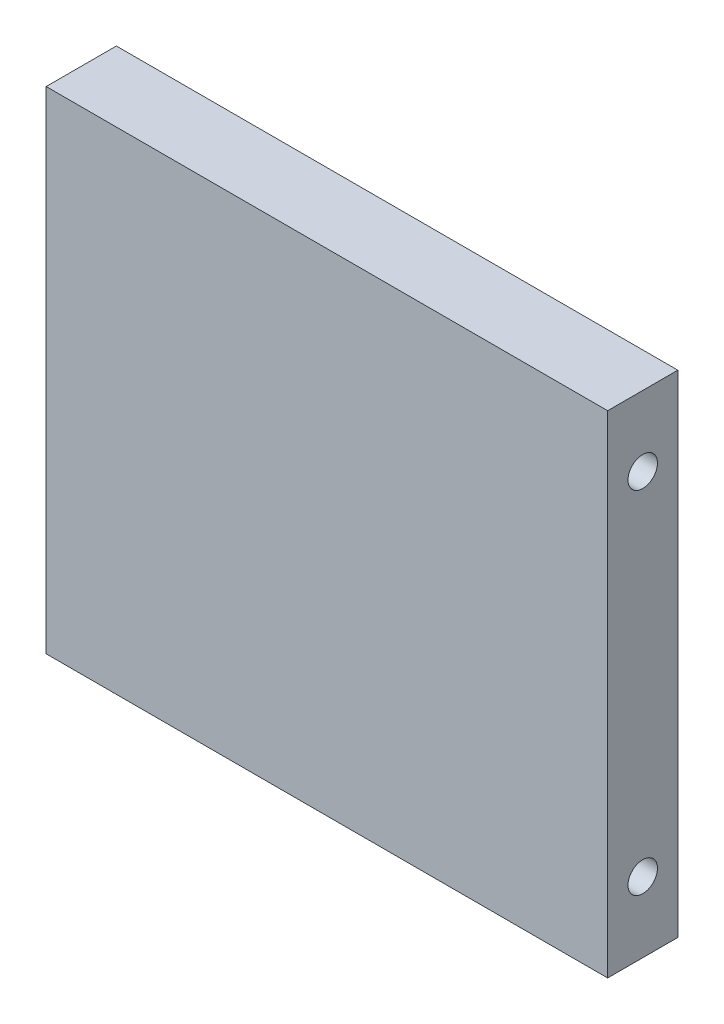
SolidWorks part; units mm, degrees
ref_plane "前视" through (0, 0, 0) normal (0, 0, 1) x (1, 0, 0)
ref_plane "上视" through (0, 0, 0) normal (0, 1, 0) x (1, 0, 0)
ref_plane "右视" through (0, 0, 0) normal (1, 0, 0) x (0, 0, -1)
sketch "草图1" plane through (0, 0, 0) normal (0, 0, 1) x (1, 0, 0)
  line L1 (-40, 35) -> (40, 35)
  line L2 (-40, 35) -> (-40, -35)
  line L3 (-40, -35) -> (40, -35)
  line L4 (40, 35) -> (40, -35)
  line L5 (-40, 35) -> (40, -35) construction
  line L6 (-40, -35) -> (40, 35) construction
  point P0 (0, 0)
  dimension "D1" = 80
  dimension "D2" = 70
extrude "凸台-拉伸1" add sketch "草图1" along normal blind 10
hole_wizard "M5 螺纹孔1" positions "草图3" profile "草图2" tap size "M5" standard "GB"
sketch "草图3" plane through (40, 0, 0) normal (1, 0, 0) x (0, 0, -1)
  line L0 (-5, -25) -> (-5, 25) construction
  line L3 (-5, 25) -> (-5, 35) construction
  line L4 (-10, 35) -> (0, 35) construction
  line L7 (-5, 0) -> (0, 0) construction
  line L8 (0, -35) -> (0, 35) construction
  point P0 (-5, -25)
  point P2 (-5, 25)
  dimension "D1" = 50
sketch "草图2" plane through (40, -25, 5) normal (0, 1, 0) x (0, 0, -1)
  line L0 (0, 0) -> (0, 15.2618)
  line L1 (0, 15.2618) -> (2.1, 14)
  line L2 (2.1, 14) -> (2.1, 0)
  line L5 (2.1, 0) -> (0, 0)
  line L10 (0, 15.2618) -> (-2.1, 14) construction
  line L11 (0, -6.35) -> (0, 107.95) construction
  dimension "螺纹孔钻头直径" = 4.2
  dimension "螺纹孔钻头深度" = 14
  dimension "导头角度" = 118
cosmetic thread "孔螺蚊线1"
cosmetic thread "孔螺蚊线2"
hole_wizard "M5 螺纹孔2" positions "草图5" profile "草图4" tap size "M5" standard "GB"
sketch "草图5" plane through (-40, 0, 0) normal (-1, 0, 0) x (0, 0, 1)
  point P0 (5, 25)
  point P3 (5, -25)
sketch "草图4" plane through (-40, 25, 5) normal (0, 1, 0) x (0, 0, 1)
  line L0 (0, 0) -> (0, 15.2618)
  line L1 (0, 15.2618) -> (2.1, 14)
  line L2 (2.1, 14) -> (2.1, 0)
  line L5 (2.1, 0) -> (0, 0)
  line L10 (0, 15.2618) -> (-2.1, 14) construction
  line L11 (0, -6.35) -> (0, 107.95) construction
  dimension "螺纹孔钻头直径" = 4.2
  dimension "螺纹孔钻头深度" = 14
  dimension "导头角度" = 118
cosmetic thread "孔螺蚊线3"
cosmetic thread "孔螺蚊线4"
